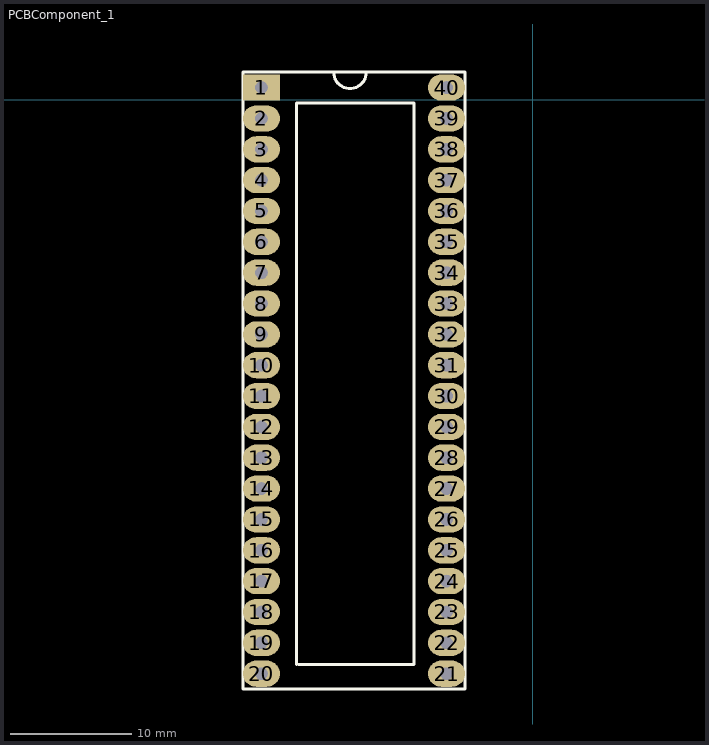
[diagram p0: the footprint, top view; thin cyan lines are the x and y axes]
# Altium footprint library MISC80722-5.PcbLib: 1 footprints
Each footprint in its own frame and in the unit in brackets; x right, y up, seen from the top. Pads: shape width x height; smd on the part's side, far side on the other; paste and mask are expansions set on the pad; w line width, h text height; cw(c..) or ccw(c..) is an arc to the next point about the centre after c.

## PCBComponent_1 [mil]
pads (40):
  rect 120x85 hole 40 slot 40.2 at 0 deg paste+0 mask+2: 1(-880,40)
  oval 120x85 hole 40 slot 40.2 at 0 deg paste+0 mask+2: 2(-880,-60) 3(-880,-160) 4(-880,-260) 5(-880,-360) 6(-880,-460) 7(-880,-560) 8(-880,-660) 9(-880,-760) 10(-880,-860) 11(-880,-960) 12(-880,-1060) 13(-880,-1160) 14(-880,-1260) 15(-880,-1360) 16(-880,-1460) 17(-880,-1560) 18(-880,-1660) 19(-880,-1760) 20(-880,-1860) 21(-280,-1860) 22(-280,-1760) 23(-280,-1660) 24(-280,-1560) 25(-280,-1460) 26(-280,-1360) 27(-280,-1260) 28(-280,-1160) 29(-280,-1060) 30(-280,-960) 31(-280,-860) 32(-280,-760) 33(-280,-660) 34(-280,-560) 35(-280,-460) 36(-280,-360) 37(-280,-260) 38(-280,-160) 39(-280,-60) 40(-280,40)
Top Overlay:
  lines w10: -765.98,-1830 -765.98,-10 -385.98,-10 -385.98,-1830 -760,-1830 ; -646,90 ccw(c-593,90) -540,90 ; -940,-1910 -220,-1910 -220,90 -940,90 -940,-1910